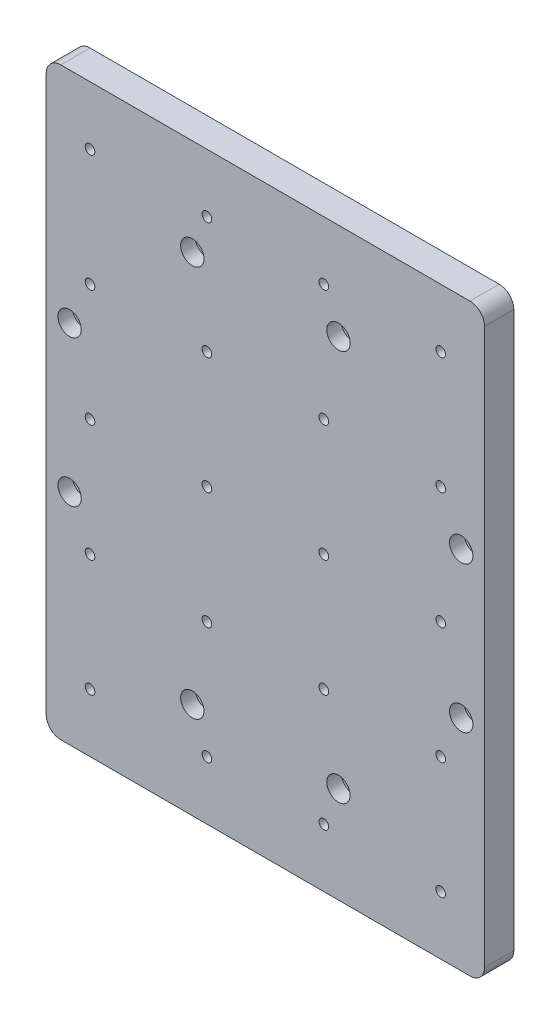
from build123d import *

# Parameters (mm, degrees)
SKETCH_1_W                  = 150
SKETCH_1_H                  = 200
SKETCH_1_R                  = 2
EXTRUDE_1_DEPTH             = 5
SKETCH_2_R                  = 4
CUT_EXTRUDE_1_DEPTH         = 4.5
HOLE_WIZARD_M4_1_D          = 3.3
HOLE_WIZARD_1_D             = 4.5
HOLE_WIZARD_1_CBORE_D       = 8
HOLE_WIZARD_1_CBORE_DEPTH   = 5
SKETCH_7_R                  = 4.920568007
SKETCH_7_R_2                = 5.393736445
SKETCH_7_R_3                = 5.34126294
SKETCH_7_R_4                = 5.362446972
EXTRUDE_2_DEPTH             = 10
FILLET_1_R                  = 5
HOLE_WIZARD_2_D             = 4.5
HOLE_WIZARD_2_CBORE_D       = 8
HOLE_WIZARD_2_CBORE_DEPTH   = 5
PATTERN_LINEAR_2_COUNT      = 4
PATTERN_LINEAR_2_PITCH      = 40
PATTERN_LINEAR_2_COUNT_DIR2 = 5
PATTERN_LINEAR_2_PITCH_DIR2 = 40


with BuildPart() as part:
    # 草图1 → 凸台-拉伸1 (new, symmetric)
    with BuildSketch(Plane.XY):
        Rectangle(SKETCH_1_W, SKETCH_1_H)
        with Locations((-67, 25)):
            Circle(SKETCH_1_R, mode=Mode.SUBTRACT)
        with Locations(Location((-67, -25, 0), (0, 0, 180))):
            Circle(SKETCH_1_R, mode=Mode.SUBTRACT)
        with Locations((67, -25)):
            Circle(SKETCH_1_R, mode=Mode.SUBTRACT)
        with Locations(Location((67, 25, 0), (0, 0, 180))):
            Circle(SKETCH_1_R, mode=Mode.SUBTRACT)
    extrude(amount=EXTRUDE_1_DEPTH, both=True)

    # 草图2 → 切除-拉伸1 (cut)
    with BuildSketch(Plane.XY.offset(5)):
        with Locations((67, 25)):
            Circle(SKETCH_2_R)
        with Locations((67, -25)):
            Circle(SKETCH_2_R)
        with Locations((-67, -25)):
            Circle(SKETCH_2_R)
        with Locations((-67, 25)):
            Circle(SKETCH_2_R)
    extrude(amount=-CUT_EXTRUDE_1_DEPTH, mode=Mode.SUBTRACT)

    # M4 螺纹孔1 (through all)
    with Locations(Plane.XY.offset(5)):
        with Locations((-60, 80)):
            hole_wizard_m4_1 = Hole(HOLE_WIZARD_M4_1_D / 2)

    # 打孔尺寸(%根据)开槽圆柱头螺钉的类型1 (through all)
    with Locations(Plane.XY.offset(5)):
        with Locations((-25, 67), (25, 67), (-25, -67), (25, -67)):
            CounterBoreHole(HOLE_WIZARD_1_D / 2, HOLE_WIZARD_1_CBORE_D / 2, HOLE_WIZARD_1_CBORE_DEPTH)

    # 草图7 → 凸台-拉伸2 (add)
    with BuildSketch(Plane.XY.offset(5)):
        with Locations((-67, 25)):
            Circle(SKETCH_7_R)
        with Locations((-67, -25)):
            Circle(SKETCH_7_R_2)
        with Locations((67, -25)):
            Circle(SKETCH_7_R_3)
        with Locations((67, 25)):
            Circle(SKETCH_7_R_4)
    extrude(amount=-EXTRUDE_2_DEPTH)

    # 圆角1
    fillet_1_edges = [part.edges().sort_by_distance(p)[0] for p in [
        (75, -100, 0),
        (-75, -100, 0),
        (-75, 100, 0),
        (75, 100, 0),
    ]]
    fillet(fillet_1_edges, radius=FILLET_1_R)

    # 打孔尺寸(%根据)开槽圆柱头螺钉的类型2 (through all)
    with Locations(Plane.XY.offset(5)):
        with Locations((-67, 25), (67, 25), (-67, -25), (67, -25)):
            CounterBoreHole(HOLE_WIZARD_2_D / 2, HOLE_WIZARD_2_CBORE_D / 2, HOLE_WIZARD_2_CBORE_DEPTH)

    # 阵列(线性)2: Hole Wizard M4 _1 4 × 5
    with Locations(*[(i * PATTERN_LINEAR_2_PITCH, -j * PATTERN_LINEAR_2_PITCH_DIR2, 0) for i in range(PATTERN_LINEAR_2_COUNT) for j in range(PATTERN_LINEAR_2_COUNT_DIR2) if (i, j) != (0, 0)]):
        add(hole_wizard_m4_1, mode=Mode.SUBTRACT)


solid = part.part
